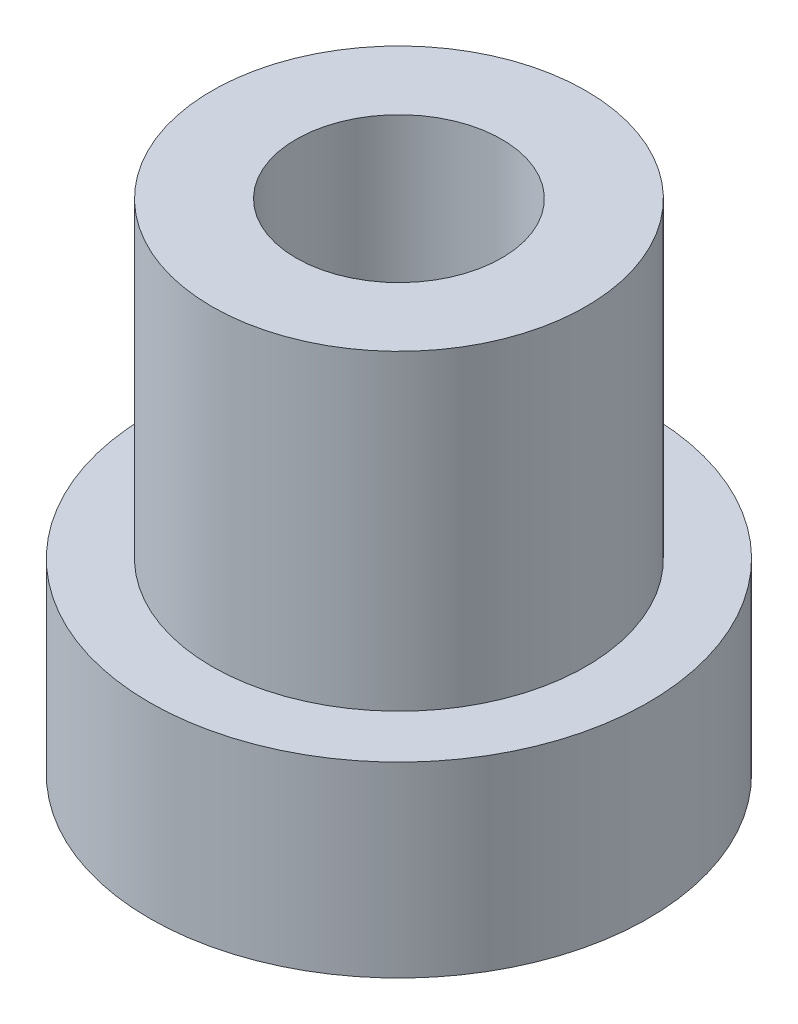
from build123d import *

# Parameters (mm, degrees)
M4_TAPPED_HOLE1_D = 3.3


with BuildPart() as part:
    # Sketch1 → Revolve1 (revolve)
    with BuildSketch(Plane.XY, mode=Mode.PRIVATE) as revolve1_sk:
        Polygon((3, 0), (3, -5), (4, -5), (4, -8), (0, -8), (0, 0), align=None)
    revolve(revolve1_sk.sketch.rotate(Axis((0, 0, 0), (0, -1, 0)), 90), axis=Axis((0, 0, 0), (0, -1, 0)))

    # M4 Tapped Hole1 (through all)
    with Locations(Plane.ZX):
        with Locations((0, 0)):
            Hole(M4_TAPPED_HOLE1_D / 2)


solid = part.part
